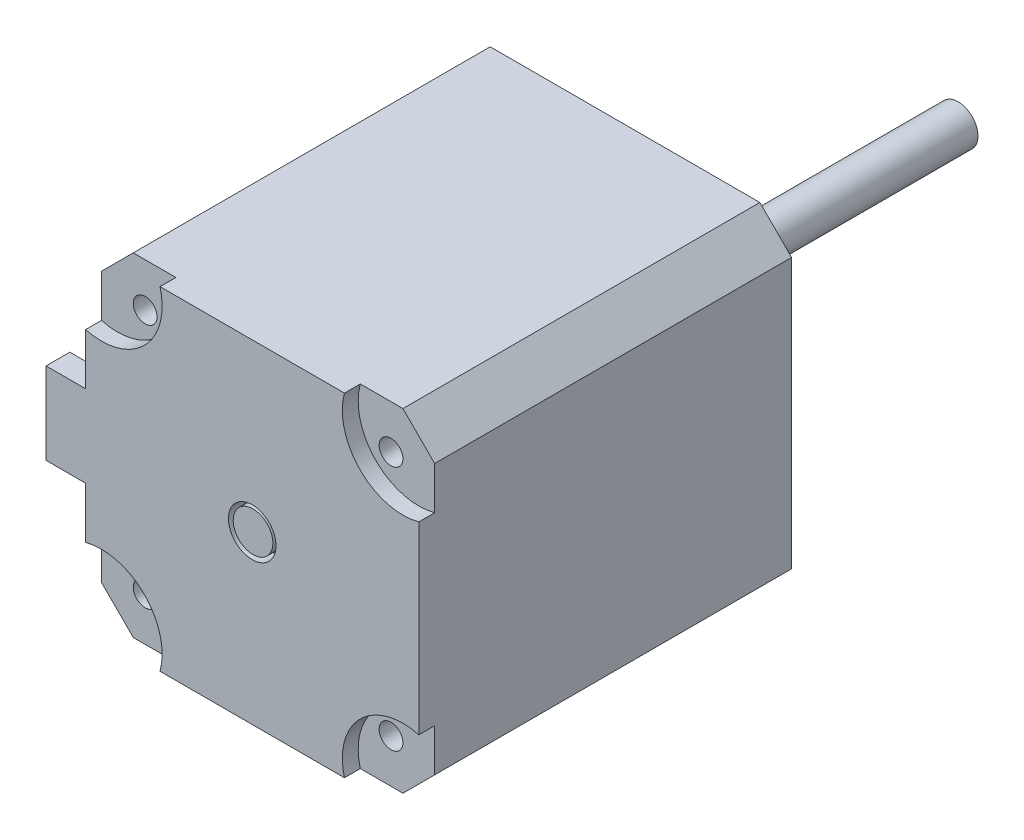
from build123d import *

# Parameters (mm, degrees)
SKETCH1_W           = 42
SKETCH1_H           = 42
SKETCH1_R           = 1.5
BOSS_EXTRUDE1_DEPTH = 47
CUT_EXTRUDE1_DEPTH  = 56.596762496
SKETCH4_R           = 11
BOSS_EXTRUDE2_DEPTH = 2
BOSS_EXTRUDE3_DEPTH = 40
CUT_EXTRUDE2_DEPTH  = 2
SKETCH8_R           = 3
CUT_EXTRUDE3_DEPTH  = 2
BOSS_EXTRUDE4_START = 1.9
SKETCH9_R           = 2.5
BOSS_EXTRUDE4_DEPTH = 1.9
SKETCH10_W          = 3
SKETCH10_H          = 10.31009041
SKETCH10_W_2        = 2.478607588
SKETCH10_H_2        = 8.518222776
BOSS_EXTRUDE5_DEPTH = 5
SKETCH11_R          = 0.5
BOSS_EXTRUDE6_DEPTH = 5


with BuildPart() as part:
    # Sketch1 → Boss-Extrude1 (new body)
    with BuildSketch(Plane.XY):
        Rectangle(SKETCH1_W, SKETCH1_H)
        with Locations((-15.5, 15.5)):
            Circle(SKETCH1_R, mode=Mode.SUBTRACT)
        with Locations(Location((15.5, 15.5, 0), (0, 0, 180))):
            Circle(SKETCH1_R, mode=Mode.SUBTRACT)
        with Locations(Location((-15.5, -15.5, 0), (0, 0, 180))):
            Circle(SKETCH1_R, mode=Mode.SUBTRACT)
        with Locations((15.5, -15.5)):
            Circle(SKETCH1_R, mode=Mode.SUBTRACT)
    extrude(amount=BOSS_EXTRUDE1_DEPTH)

    # Sketch3 → Cut-Extrude1 (cut, through all)
    with BuildSketch(Plane(origin=(0, 0, 0), x_dir=(-1, 0, 0), z_dir=(0, 0, -1))):
        Polygon((-21, 17), (-17, 21), (-21, 21), align=None)
        Polygon((21, 21), (17, 21), (21, 17), align=None)
        Polygon((21, -17), (17, -21), (21, -21), align=None)
        Polygon((-21, -21), (-17, -21), (-21, -17), align=None)
    extrude(amount=-CUT_EXTRUDE1_DEPTH, mode=Mode.SUBTRACT)

    # Sketch4 → Boss-Extrude2 (add)
    with BuildSketch(Plane(origin=(0, 0, 0), x_dir=(-1, 0, 0), z_dir=(0, 0, -1))):
        Circle(SKETCH4_R)
    extrude(amount=BOSS_EXTRUDE2_DEPTH)

    # Sketch5 → Boss-Extrude3 (add)
    with BuildSketch(Plane(origin=(0, 0, -2), x_dir=(-1, 0, 0), z_dir=(0, 0, -1))):
        with BuildLine():
            Line((1.7, -1.833030278), (1.7, 1.833030278))
            ThreePointArc((1.7, 1.833030278), (-2.5, 0), (1.7, -1.833030278))
        make_face()
    extrude(amount=BOSS_EXTRUDE3_DEPTH)

    # Sketch7 → Cut-Extrude2 (cut)
    with BuildSketch(Plane.XY.offset(47)):
        with BuildLine():
            Line((21, 17), (21, 11.625484678))
            ThreePointArc((21, 11.625484678), (13.597062084, 13.597062084), (11.625484678, 21))
            Line((11.625484678, 21), (17, 21))
            Line((17, 21), (21, 17))
        make_face()
        with BuildLine():
            Line((-21, -17), (-21, -11.625484678))
            ThreePointArc((-21, -11.625484678), (-13.597062084, -13.597062084), (-11.625484678, -21))
            Line((-11.625484678, -21), (-17, -21))
            Line((-17, -21), (-21, -17))
        make_face()
        with BuildLine():
            Line((-11.625484678, 21), (-17, 21))
            Line((-17, 21), (-21, 17))
            Line((-21, 17), (-21, 11.625484678))
            ThreePointArc((-21, 11.625484678), (-13.597062084, 13.597062084), (-11.625484678, 21))
        make_face()
        with BuildLine():
            Line((11.625484678, -21), (17, -21))
            Line((17, -21), (21, -17))
            Line((21, -17), (21, -11.625484678))
            ThreePointArc((21, -11.625484678), (13.597062084, -13.597062084), (11.625484678, -21))
        make_face()
    extrude(amount=-CUT_EXTRUDE2_DEPTH, mode=Mode.SUBTRACT)

    # Sketch8 → Cut-Extrude3 (cut)
    with BuildSketch(Plane.XY.offset(47)):
        Circle(SKETCH8_R)
    extrude(amount=-CUT_EXTRUDE3_DEPTH, mode=Mode.SUBTRACT)

    # Sketch9 → Boss-Extrude4 (add)
    with BuildSketch(Plane.XY.offset(45).offset(BOSS_EXTRUDE4_START)):
        with Locations(Location((0, 0, 0), (0, 0, 180))):
            Circle(SKETCH9_R)
    extrude(amount=-BOSS_EXTRUDE4_DEPTH)

    # Sketch10 → Boss-Extrude5 (add)
    with BuildSketch(Plane.ZY.offset(21)):
        with Locations((45.5, 0)):
            Rectangle(SKETCH10_W, SKETCH10_H)
        with Locations((45.5, 0)):
            Rectangle(SKETCH10_W_2, SKETCH10_H_2, mode=Mode.SUBTRACT)
    extrude(amount=BOSS_EXTRUDE5_DEPTH)

    # Sketch11 → Boss-Extrude6 (add)
    with BuildSketch(Plane.ZY.offset(21)):
        with Locations(Location((45.5, 3.127782029, 0), (0, 0, 180))):
            Circle(SKETCH11_R)
        with Locations(Location((45.5, 1.627782029, 0), (0, 0, 180))):
            Circle(SKETCH11_R)
        with Locations(Location((45.5, 0.127782029, 0), (0, 0, 180))):
            Circle(SKETCH11_R)
        with Locations(Location((45.5, -1.372217971, 0), (0, 0, 180))):
            Circle(SKETCH11_R)
        with Locations(Location((45.5, -2.872217971, 0), (0, 0, 180))):
            Circle(SKETCH11_R)
    extrude(amount=BOSS_EXTRUDE6_DEPTH)


solid = part.part
